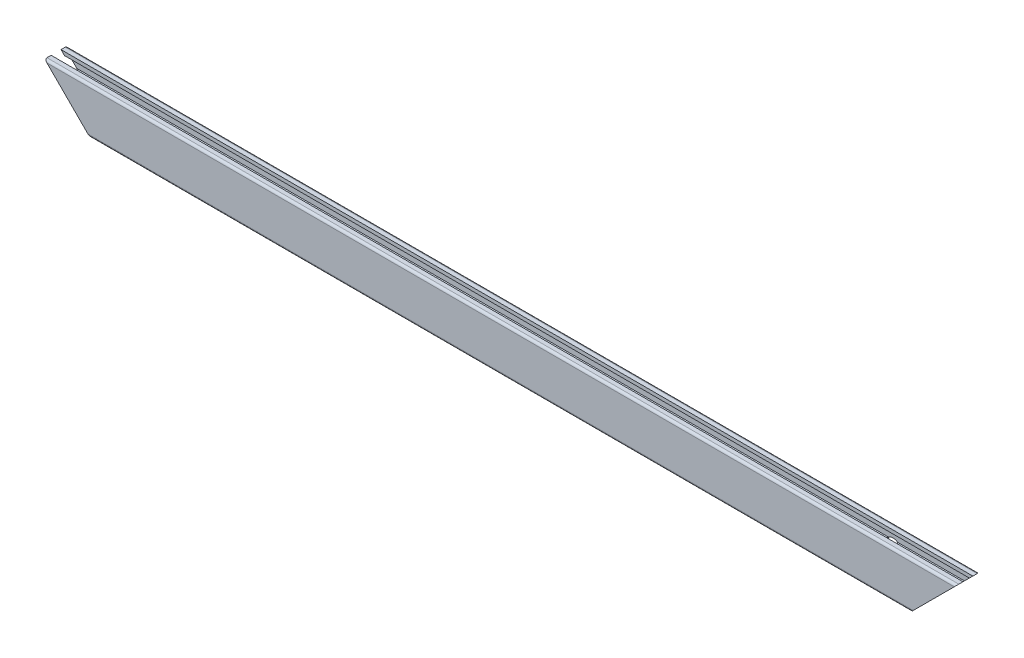
from build123d import *

# Parameters (mm, degrees)
SKETCH12_R          = 2.5
MEMBER_1_DEPTH      = 600
CUT_EXTRUDE_1_DEPTH = 301.749064836
SKETCH_7_R          = 5
CUT_EXTRUDE_2_DEPTH = 4.999


with BuildPart() as part:
    # Sketch12 → Member 1 (new body)
    with BuildSketch(Plane(origin=(-300, 0, 0), x_dir=(0, 0, -1), z_dir=(1, 0, 0))):
        with BuildLine():
            Line((-6, -15), (-3.25, -15))
            Line((-3.25, -15), (-3.25, -12.7))
            Line((-3.25, -12.7), (-5.7, -12.7))
            Line((-5.7, -12.7), (-5.7, -7))
            ThreePointArc((-5.7, -7), (0, -4.5), (5.7, -7))
            Line((5.7, -7), (5.7, -12.7))
            Line((5.7, -12.7), (3.25, -12.7))
            Line((3.25, -12.7), (3.25, -15))
            Line((3.25, -15), (6, -15))
            ThreePointArc((6, -15), (7.060660172, -14.560660172), (7.5, -13.5))
            Line((7.5, -13.5), (7.5, 13.5))
            ThreePointArc((7.5, 13.5), (7.060660172, 14.560660172), (6, 15))
            Line((6, 15), (3.25, 15))
            Line((3.25, 15), (3.25, 12.7))
            Line((3.25, 12.7), (5.7, 12.7))
            Line((5.7, 12.7), (5.7, 7))
            ThreePointArc((5.7, 7), (0, 4.5), (-5.7, 7))
            Line((-5.7, 7), (-5.7, 12.7))
            Line((-5.7, 12.7), (-3.25, 12.7))
            Line((-3.25, 12.7), (-3.25, 15))
            Line((-3.25, 15), (-6, 15))
            ThreePointArc((-6, 15), (-7.060660172, 14.560660172), (-7.5, 13.5))
            Line((-7.5, 13.5), (-7.5, -13.5))
            ThreePointArc((-7.5, -13.5), (-7.060660172, -14.560660172), (-6, -15))
        make_face()
        Circle(SKETCH12_R, mode=Mode.SUBTRACT)
    extrude(amount=MEMBER_1_DEPTH)

    # 草图4 → 切除-拉伸1 (cut, through all)
    with BuildSketch(Plane.XY.offset(7.5)):
        Polygon((-300, 15), (-270, -15), (-300, -15), align=None)
        Polygon((300, -15), (300, 15), (270, -15), align=None)
    extrude(amount=-CUT_EXTRUDE_1_DEPTH, mode=Mode.SUBTRACT)

    # 草图7 → 切除-拉伸2 (cut)
    with BuildSketch(Plane.XY.offset(-7.5)):
        with Locations(Location((245, 3, 0), (0, 0, 157.483422962))):
            Circle(SKETCH_7_R)
    extrude(amount=CUT_EXTRUDE_2_DEPTH, mode=Mode.SUBTRACT)


solid = part.part
